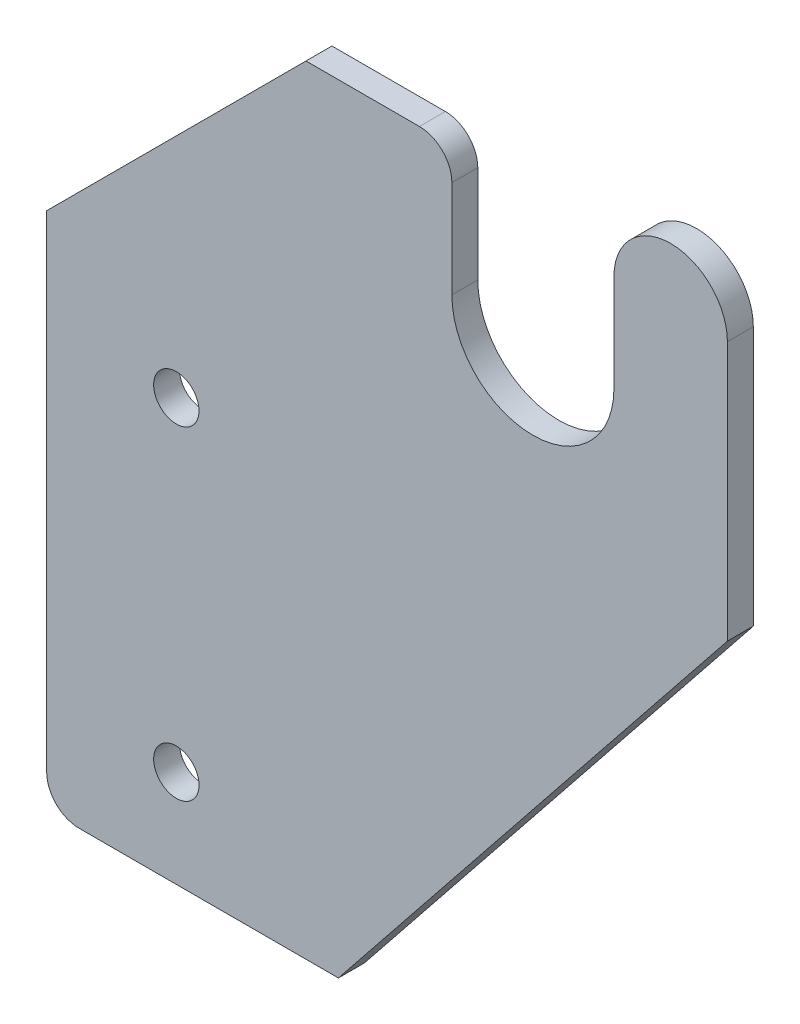
from build123d import *

# Parameters (mm, degrees)
SKETCH1_R           = 7
BOSS_EXTRUDE1_DEPTH = 8


with BuildPart() as part:
    # Sketch1 → Boss-Extrude1 (new body)
    with BuildSketch(Plane.XY):
        with BuildLine():
            Line((10, 0), (90, 0))
            Line((90, 0), (210, 150))
            Line((210, 150), (210, 230))
            ThreePointArc((210, 230), (192.5, 247.5), (175, 230))
            Line((175, 230), (175, 200))
            ThreePointArc((175, 200), (150, 175), (125, 200))
            Line((125, 200), (125, 230))
            ThreePointArc((125, 230), (122.071067812, 237.071067812), (115, 240))
            Line((115, 240), (80, 240))
            Line((80, 240), (0, 160))
            Line((0, 160), (0, 10))
            ThreePointArc((0, 10), (2.928932188, 2.928932188), (10, 0))
        make_face()
        with Locations((40, 130)):
            Circle(SKETCH1_R, mode=Mode.SUBTRACT)
        with Locations((40, 30)):
            Circle(SKETCH1_R, mode=Mode.SUBTRACT)
    extrude(amount=BOSS_EXTRUDE1_DEPTH)


solid = part.part
